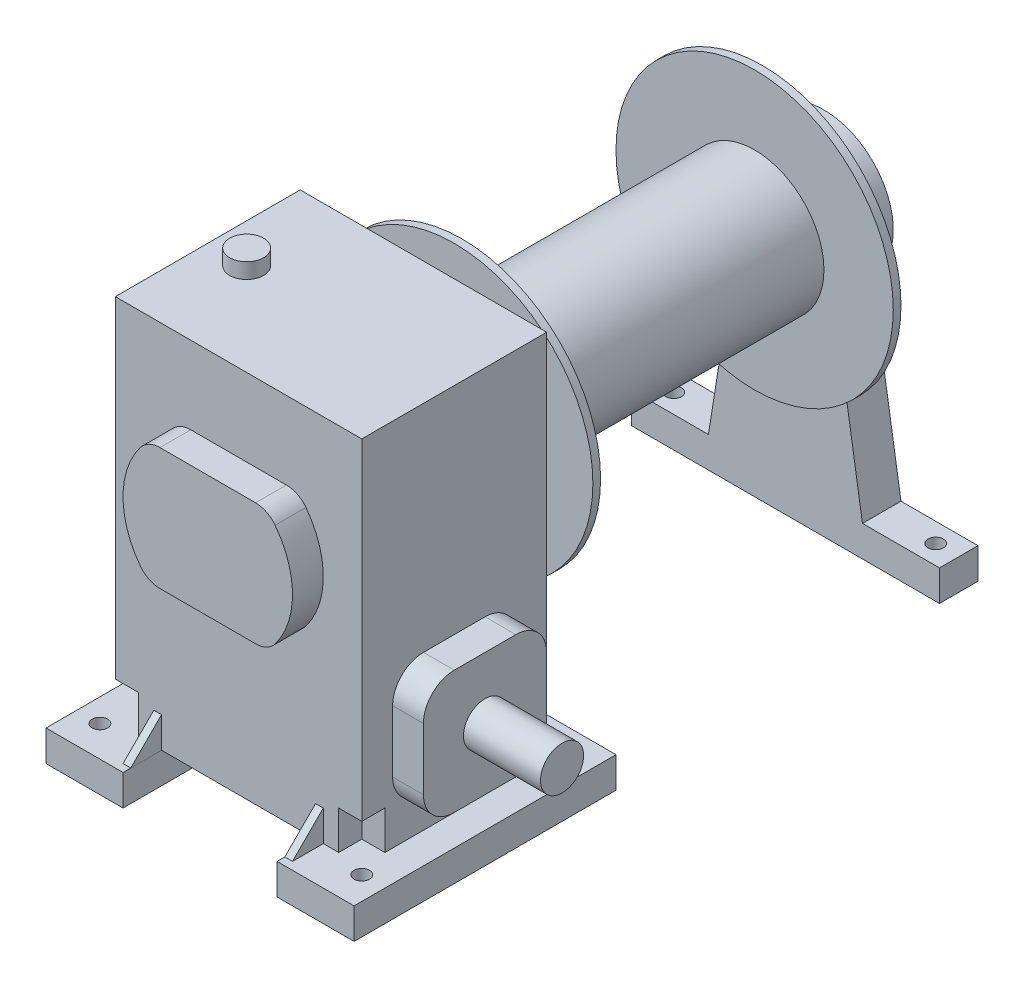
SolidWorks part; units mm, degrees
ref_plane "前视基准面" through (0, 0, 0) normal (0, 0, 1) x (1, 0, 0)
ref_plane "上视基准面" through (0, 0, 0) normal (0, 1, 0) x (1, 0, 0)
ref_plane "右视基准面" through (0, 0, 0) normal (1, 0, 0) x (0, 0, -1)
sketch "草图1" plane through (0, 0, 0) normal (1, 0, 0) x (0, 0, -1)
  line L0 (-92.4228, 0) -> (105.6221, 0)
  line L1 (105.6221, 0) -> (105.6221, 90)
  line L2 (105.6221, 90) -> (100.6221, 90)
  line L3 (100.6221, 90) -> (100.6221, 45)
  line L4 (100.6221, 45) -> (-89.3779, 45)
  line L5 (-89.3779, 45) -> (-89.3779, 90)
  line L6 (-89.3779, 90) -> (-94.3779, 90)
  line L7 (-94.3779, 90) -> (-94.3779, 0)
  line L8 (-94.3779, 0) -> (-92.4228, 0)
  line L9 (-1000, 0) -> (49000, 0) construction
  dimension "D1" = 200
  dimension "D2" = 5
  dimension "D3" = 45
  dimension "D4" = 90
  dimension "D6" = 5
revolve "旋转1" add sketch "草图1" angle 360 about L9
sketch "草图2" plane through (0, 0, 94.3779) normal (0, 0, 1) x (1, 0, 0)
  circle A0 centre (0, 0) radius 10
  dimension "D1" = 20
extrude "凸台-拉伸1" add sketch "草图2" along normal blind 20 and the other way blind 240
sketch "草图3" plane through (0, 0, 114.3779) normal (0, 0, 1) x (1, 0, 0)
  line L0 (0, -150) -> (0, 90) construction
  line L1 (-80, 90) -> (80, 90)
  line L2 (-80, 90) -> (-80, -150)
  line L3 (-80, -150) -> (80, -150)
  line L4 (80, 90) -> (80, -150)
  point P0 (0, 0)
  dimension "D1" = 160
  dimension "D2" = 90
  dimension "D3" = 240
extrude "凸台-拉伸2" add sketch "草图3" along normal blind 120
sketch "草图4" plane through (0, 0, -145.6221) normal (0, 0, -1) x (-1, 0, 0)
  line L1 (-50, -150) -> (-100, -150)
  line L2 (-100, -150) -> (-100, -170)
  line L3 (100, -150) -> (100, -170)
  line L4 (50, -150) -> (100, -150)
  line L6 (-100, -170) -> (100, -170)
  line L7 (0, 0) -> (0, -65.9934) construction
  line L8 (-50, -150) -> (-31.2119, -32.4163)
  line L9 (50, -150) -> (31.2119, -32.4163)
  arc A0 (45, 0) -> (-45, 0) centre (0, 0) ccw
  circle A1 centre (0, 0) radius 10
  arc A2 (45, 0) -> (31.2119, -32.4163) centre (0, 0) cw
  arc A3 (-31.2119, -32.4163) -> (-45, 0) centre (0, 0) cw
  dimension "D1" = 170
  dimension "D4" = 45
  dimension "D2" = 200
  dimension "D3" = 20
  dimension "D5" = 50
extrude "凸台-拉伸3" add sketch "草图4" against normal blind 25 separate body
sketch "草图6" plane through (0, 0, 234.3779) normal (0, 0, 1) x (1, 0, 0)
  line L0 (-38.1475, 39.6203) -> (38.1475, 39.6203)
  line L1 (-38.1475, -39.6203) -> (38.1475, -39.6203)
  arc A0 (-38.1475, 39.6203) -> (-38.1475, -39.6203) centre (0, 0) ccw
  arc A1 (38.1475, -39.6203) -> (38.1475, 39.6203) centre (0, 0) ccw
extrude "凸台-拉伸4" add sketch "草图6" along normal blind 20
sketch "草图7" plane through (80, 0, 0) normal (1, 0, 0) x (0, 0, -1)
  line L0 (-234.3779, -150) -> (-114.3779, -150) construction
  line L1 (-214.3779, -130) -> (-134.3779, -130)
  line L2 (-214.3779, -130) -> (-214.3779, -50)
  line L3 (-214.3779, -50) -> (-134.3779, -50)
  line L4 (-134.3779, -130) -> (-134.3779, -50)
  line L5 (-214.3779, -130) -> (-134.3779, -50) construction
  line L6 (-214.3779, -50) -> (-134.3779, -130) construction
  line L7 (-174.3779, 90) -> (-174.3779, 31.9374) construction
  line L8 (-234.3779, 90) -> (-114.3779, 90) construction
  point P0 (-174.3779, -90)
  dimension "D1" = 60
  dimension "D2" = 80
  dimension "D3" = 80
extrude "凸台-拉伸5" add sketch "草图7" along normal blind 20 and the other way blind 180
fillet "圆角1" radius 20 8 edges at (90, -130, 214.3779) (90, -130, 134.3779) (90, -50, 134.3779) (90, -50, 214.3779) (-90, -130, 134.3779) (-90, -130, 214.3779) (-90, -50, 134.3779) (-90, -50, 214.3779)
fillet "圆角2" radius 16 4 edges at (-38.1475, -39.6203, 244.3779) (38.1475, -39.6203, 244.3779) (-38.1475, 39.6203, 244.3779) (38.1475, 39.6203, 244.3779)
sketch "草图8" plane through (100, 0, 0) normal (1, 0, 0) x (0, 0, -1)
  line L0 (-214.3779, -90) -> (-134.3779, -90) construction
  line L2 (-214.3779, -70) -> (-214.3779, -110) construction
  line L3 (-134.3779, -70) -> (-134.3779, -110) construction
  circle A0 centre (-174.3779, -90) radius 14
extrude "凸台-拉伸6" add sketch "草图8" along normal blind 50
ref_plane "基准面1" through (0, 0, 174.3779) normal (0, 0, 1) x (1, 0, 0)
sketch "草图10" plane through (0, 0, 174.3779) normal (0, 0, 1) x (1, 0, 0)
  line L0 (50, -150) -> (100, -150) construction
  line L1 (50, -150) -> (100, -150)
  line L2 (50, -150) -> (50, -170)
  line L3 (50, -170) -> (100, -170)
  line L4 (100, -150) -> (100, -170)
  line L5 (-100, -150) -> (-50, -150) construction
  line L6 (-100, -170) -> (-50, -170)
  line L7 (-100, -170) -> (-100, -150)
  line L8 (-100, -150) -> (-50, -150)
  line L9 (-50, -170) -> (-50, -150)
  dimension "D1" = 50
extrude "凸台-拉伸7" add sketch "草图10" along normal mid plane 170 separate body
sketch "草图11" plane through (50, 0, 0) normal (-1, 0, 0) x (0, 0, 1)
  line L0 (114.3779, -130) -> (94.3779, -150)
  line L1 (114.3779, 90) -> (114.3779, -150) construction
  line L2 (259.3779, -150) -> (89.3779, -150) construction
  line L3 (94.3779, -150) -> (114.3779, -150)
  line L4 (114.3779, -130) -> (114.3779, -150)
  line L6 (234.3779, -150) -> (114.3779, -150) construction
  line L7 (174.3779, -99.7819) -> (174.3779, -120.4509) construction
  line L8 (174.3779, -88) -> (174.3779, 88) construction
  line L9 (234.3779, -130) -> (234.3779, -150)
  line L10 (234.3779, -130) -> (254.3779, -150)
  line L11 (234.3779, -150) -> (254.3779, -150)
  point P17 (174.3779, -150)
  point P18 (174.3779, -150)
  dimension "D1" = 20
  dimension "D2" = 160
extrude "凸台-拉伸8" add sketch "草图11" against normal blind 5
mirror "镜向1" about plane through (0, 0, 0) normal (1, 0, 0) of "凸台-拉伸8"
sketch "草图12" plane through (0, -170, 0) normal (0, -1, 0) x (1, 0, 0)
  line L0 (-100, 174.3779) -> (180.3339, 174.3779) construction
  line L1 (-100, 259.3779) -> (-100, 89.3779) construction
  line L2 (88, 174.3779) -> (-88, 174.3779) construction
  line L3 (0, 298.914) -> (0, -185.6839) construction
  circle A0 centre (85, 239.3779) radius 5
  circle A1 centre (85, 109.3779) radius 5
  circle A2 centre (85, -133.1221) radius 5
  circle A3 centre (-85, -133.1221) radius 5
  circle A4 centre (-85, 109.3779) radius 5
  circle A5 centre (-85, 239.3779) radius 5
  dimension "D1" = 10
  dimension "D2" = 170
  dimension "D3" = 130
extrude "切除-拉伸1" cut sketch "草图12" against normal up to next (20 mm away)
sketch "草图13" plane through (0, -150, 0) normal (0, -1, 0) x (1, 0, 0)
  line L0 (-70.579, 174.3779) -> (145.4232, 174.3779) construction
  line L1 (-80, 234.3779) -> (-65, 234.3779)
  line L2 (-80, 234.3779) -> (-80, 219.3779)
  line L3 (-80, 219.3779) -> (-65, 219.3779)
  line L4 (-65, 234.3779) -> (-65, 219.3779)
  line L5 (88, 174.3779) -> (-88, 174.3779) construction
  line L6 (0, 234.3779) -> (0, 150.9228) construction
  line L7 (-50, 234.3779) -> (50, 234.3779) construction
  line L8 (80, 219.3779) -> (65, 219.3779)
  line L9 (80, 234.3779) -> (80, 219.3779)
  line L10 (65, 234.3779) -> (65, 219.3779)
  line L11 (80, 234.3779) -> (65, 234.3779)
  line L12 (80, 129.3779) -> (65, 129.3779)
  line L13 (80, 114.3779) -> (80, 129.3779)
  line L14 (80, 114.3779) -> (65, 114.3779)
  line L15 (65, 114.3779) -> (65, 129.3779)
  line L16 (-80, 129.3779) -> (-65, 129.3779)
  line L17 (-65, 114.3779) -> (-65, 129.3779)
  line L18 (-80, 114.3779) -> (-80, 129.3779)
  line L19 (-80, 114.3779) -> (-65, 114.3779)
  dimension "D1" = 15
  dimension "D2" = 15
extrude "切除-拉伸2" cut sketch "草图13" against normal blind 25
sketch "草图14" plane through (0, 90, 0) normal (0, 1, 0) x (1, 0, 0)
  line L0 (-88, -174.3779) -> (88, -174.3779) construction
  circle A0 centre (-54.7504, -174.3779) radius 11
extrude "凸台-拉伸9" add sketch "草图14" along normal blind 10
